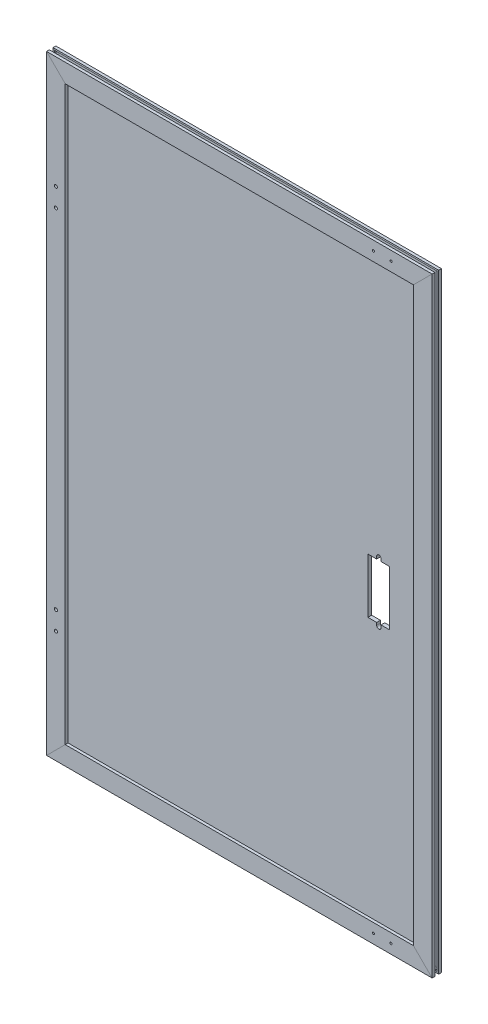
SolidWorks part; units mm, degrees
ref_plane "Front" through (0, 0, 0) normal (0, 0, 1) x (1, 0, 0)
ref_plane "Top" through (0, 0, 0) normal (0, 1, 0) x (1, 0, 0)
ref_plane "Right" through (0, 0, 0) normal (1, 0, 0) x (0, 0, -1)
sketch3d "3DSketch1"
  line L1 (294.25, 474, 0) -> (-294.25, 474, 0)
  line L2 (294.25, 474, 0) -> (294.25, -474, 0)
  line L3 (294.25, -474, 0) -> (-294.25, -474, 0)
  line L4 (-294.25, 474, 0) -> (-294.25, -474, 0)
  line L5 (294.25, 474, 0) -> (-294.25, -474, 0) construction
  line L6 (294.25, -474, 0) -> (-294.25, 474, 0) construction
  point P0 (0, 0, 0)
  dimension "D1" = 588.5
  dimension "D2" = 948
other "Aluminum profile 1530(1)"
ref_plane "Plane1" through (-294.25, 474, 0) normal (0, -1, 0) x (1, 0, 0)
sketch "Sketch1" plane through (-294.25, 474, 0) normal (0, -1, 0) x (1, 0, 0)
  line L4 (-15, -3) -> (-15, -7.5)
  line L5 (-15, -3) -> (-12.5, -3)
  line L6 (-15, -7.5) -> (15, -7.5)
  line L7 (-12.5, -3) -> (-12.5, -5)
  line L8 (15, -3) -> (15, -7.5)
  line L9 (-12.5, -5) -> (-7, -5)
  line L10 (15, -3) -> (12.5, -3)
  line L11 (-7, -5) -> (-7, -3)
  line L12 (12.5, -3) -> (12.5, -5)
  line L13 (-7, -3) -> (-4.5, -3)
  line L14 (12.5, -5) -> (7, -5)
  line L15 (-4.5, -3) -> (-4.5, 3)
  line L16 (7, -5) -> (7, -3)
  line L17 (-4.5, 3) -> (-7, 3)
  line L18 (7, -3) -> (4.5, -3)
  line L19 (-7, 3) -> (-7, 5)
  line L20 (4.5, -3) -> (4.5, 3)
  line L21 (-7, 5) -> (-12.5, 5)
  line L22 (4.5, 3) -> (7, 3)
  line L23 (-12.5, 5) -> (-12.5, 3)
  line L24 (7, 3) -> (7, 5)
  line L25 (-12.5, 3) -> (-15, 3)
  line L26 (7, 5) -> (12.5, 5)
  line L27 (-15, 7.5) -> (-15, 3)
  line L28 (12.5, 5) -> (12.5, 3)
  line L29 (15, 7.5) -> (-15, 7.5)
  line L30 (12.5, 3) -> (15, 3)
  line L31 (15, 7.5) -> (15, 3)
  circle A0 centre (0, 0) radius 2.5
  point P0 (0, 0)
other "Trim/Extend1"
other "Trim/Extend2"
other "Trim/Extend3"
other "Trim/Extend4"
sketch "Sketch2" plane through (0, 0, 0) normal (0, 0, 1) x (1, 0, 0)
  line L0 (-309.25, 489) -> (-279.25, 459) construction
  line L1 (289.25, -469) -> (-289.25, -469)
  line L2 (289.25, -469) -> (289.25, 469)
  line L3 (289.25, 469) -> (-289.25, 469)
  line L4 (-289.25, -469) -> (-289.25, 469)
  line L5 (289.25, -469) -> (-289.25, 469) construction
  line L6 (289.25, 469) -> (-289.25, -469) construction
  line L7 (-279.25, 459) -> (279.25, 459) construction
  point P0 (0, 0)
  dimension "D1" = 10
extrude "Boss-Extrude1" add sketch "Sketch2" along normal mid plane 6 separate body
sketch "Sketch3" plane through (0, 0, 3) normal (0, 0, 1) x (1, 0, 0)
  line L0 (219.25, -48) -> (219.25, 48) construction
  line L1 (201.75, -44) -> (236.75, -44)
  line L2 (201.75, -44) -> (201.75, 44)
  line L3 (201.75, 44) -> (236.75, 44)
  line L4 (236.75, -44) -> (236.75, 44)
  line L5 (201.75, -44) -> (236.75, 44) construction
  line L6 (201.75, 44) -> (236.75, -44) construction
  line L7 (215.75, -48) -> (215.75, 48)
  line L8 (222.75, -48) -> (222.75, 48)
  line L9 (219.25, 0) -> (-279.25, 0) construction
  line L10 (-279.25, -459) -> (-279.25, 459) construction
  line L11 (279.25, -459) -> (279.25, 459) construction
  arc A0 (215.75, -48) -> (222.75, -48) centre (219.25, -48) ccw
  arc A1 (222.75, 48) -> (215.75, 48) centre (219.25, 48) ccw
  point P0 (219.25, 0)
  point P7 (219.25, 0)
  dimension "D4" = 3.5
  dimension "D1" = 60
  dimension "D2" = 35
  dimension "D3" = 88
  dimension "D5" = 96
extrude "Cut-Extrude1" cut sketch "Sketch3" against normal through all contours L4 L3 L2 L1 | A1 L7 A0 L8
hole_wizard "M6 Tapped Hole1" positions "Sketch4" profile "Sketch5" tap size "M6" standard "GB" end condition through all
sketch "Sketch4" plane through (0, 0, 7.5) normal (0, 0, 1) x (1, 0, 0)
  line L0 (-294.25, 309) -> (-294.25, 279)
  line L1 (-294.25, 279) -> (-294.25, -279)
  line L2 (-294.25, -279) -> (-294.25, -309)
  line L4 (-294.25, 0) -> (0, 0)
  line L5 (-309.25, 489) -> (309.25, 489) construction
  line L6 (-309.25, -489) -> (-309.25, 489) construction
  point P0 (-294.25, 309)
  point P2 (-294.25, 279)
  point P4 (-294.25, -279)
  point P6 (-294.25, -309)
  dimension "D1" = 180
  dimension "D2" = 15
  dimension "D3" = 30
sketch "Sketch5" plane through (-294.25, 309, 7.5) normal (1, 0, 0) x (0, -1, 0)
  line L0 (0, 0) -> (0, 15)
  line L1 (0, 15) -> (2.5, 15)
  line L2 (2.5, 15) -> (2.5, 0)
  line L5 (2.5, 0) -> (0, 0)
  line L11 (0, -6.35) -> (0, 107.95) construction
  dimension "通孔螺纹孔钻头直径" = 5
  dimension "通孔螺纹孔钻头深度" = 15
cosmetic thread "Hole-Thread1" parameters "D2"=6
cosmetic thread "Hole-Thread2" parameters "D2"=6
cosmetic thread "Hole-Thread3" parameters "D2"=6
cosmetic thread "Hole-Thread4" parameters "D2"=6
hole_wizard "M4 Tapped Hole1" positions "Sketch6" profile "Sketch7" tap size "M4" standard "GB"
sketch "Sketch6" plane through (0, 0, 7.5) normal (0, 0, 1) x (1, 0, 0)
  line L1 (215.25, -474) -> (243.25, -474)
  line L2 (215.25, -474) -> (215.25, 474)
  line L3 (215.25, 474) -> (243.25, 474)
  line L4 (243.25, -474) -> (243.25, 474)
  line L5 (-309.25, -489) -> (309.25, -489) construction
  line L6 (243.25, 0) -> (309.25, 0)
  line L7 (309.25, -489) -> (309.25, 489) construction
  point P0 (215.25, 474)
  point P2 (243.25, 474)
  point P4 (215.25, -474)
  point P6 (243.25, -474)
  point P66 (229.25, 474)
  dimension "D1" = 28
  dimension "D2" = 15
  dimension "D3" = 80
sketch "Sketch7" plane through (215.25, 474, 7.5) normal (1, 0, 0) x (0, -1, 0)
  line L0 (0, 0) -> (0, 12.4914)
  line L1 (0, 12.4914) -> (1.65, 11.5)
  line L2 (1.65, 11.5) -> (1.65, 0)
  line L5 (1.65, 0) -> (0, 0)
  line L10 (0, 12.4914) -> (-1.65, 11.5) construction
  line L11 (0, -6.35) -> (0, 107.95) construction
  dimension "螺纹孔钻头直径" = 3.3
  dimension "螺纹孔钻头深度" = 11.5
  dimension "导头角度" = 118
cosmetic thread "Hole-Thread5" parameters "D1"=8, "D2"=4
cosmetic thread "Hole-Thread6" parameters "D1"=8, "D2"=4
cosmetic thread "Hole-Thread7" parameters "D1"=8, "D2"=4
cosmetic thread "Hole-Thread8" parameters "D1"=8, "D2"=4
